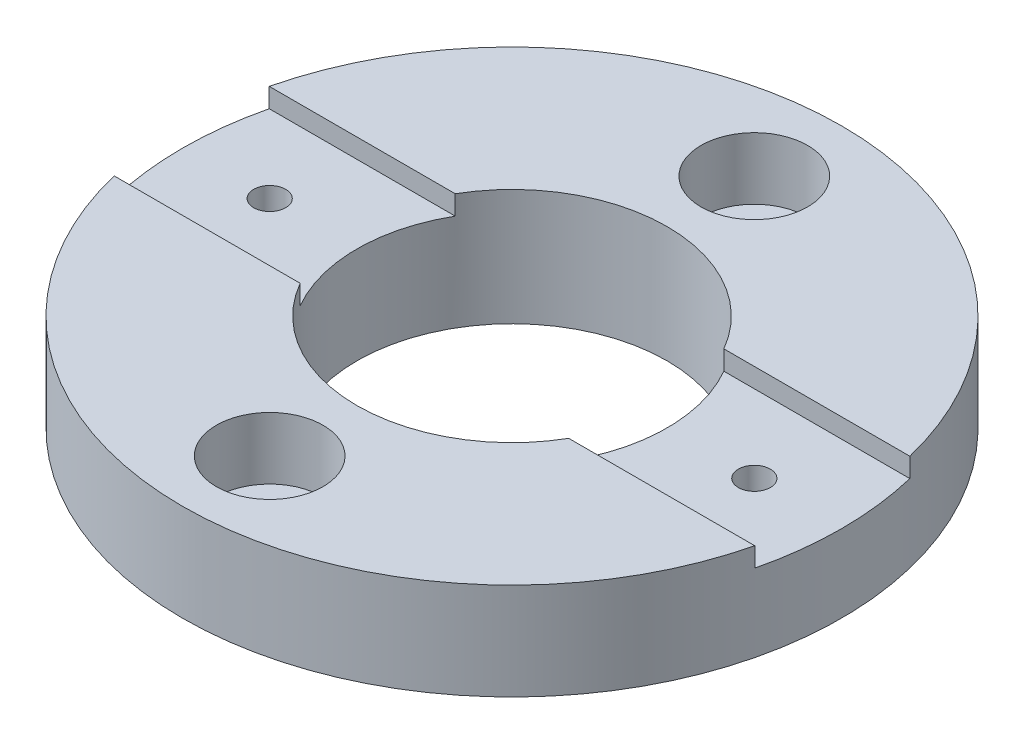
from build123d import *

# Parameters (mm, degrees)
HOLE_WIZARD_M6_1_D           = 6.6
HOLE_WIZARD_M6_1_CBORE_D     = 11
HOLE_WIZARD_M6_1_CBORE_DEPTH = 6.4
SKETCH_4_R                   = 16
CUT_EXTRUDE_1_DEPTH          = 67.543219038
EXTRUDE_1_DEPTH              = 10
SKETCH_6_W                   = 38
SKETCH_6_H                   = 16
CUT_EXTRUDE_2_DEPTH          = 10
CUT_EXTRUDE_3_DEPTH          = 74.810568349
CUT_EXTRUDE_3_DEPTH_BACK     = 74.810568349
SKETCH_7_R                   = 2
SKETCH_9_R                   = 20
CUT_EXTRUDE_5_DEPTH          = 34
SKETCH_10_W                  = 100
SKETCH_10_H                  = 16
CUT_EXTRUDE_6_DEPTH          = 12
HOLE_WIZARD_M4_1_D           = 3.3


with BuildPart() as part:
    # 草图1 → 旋转1 (revolve)
    with BuildSketch(Plane.XY, mode=Mode.PRIVATE) as revolve_1_sk:
        Polygon((0, 46), (34, 46), (34, 36), (18.4, 36), (18.4, 26), (17.492059993, 0), (0, 0), align=None)
    revolve(revolve_1_sk.sketch.rotate(Axis((0, 0, 0), (0, 1, 0)), 90), axis=Axis((0, 0, 0), (0, 1, 0)))

    # M6 六角凹头螺钉的柱形沉头孔1 (through all)
    with Locations(Plane(origin=(0, 46, 0), x_dir=(1, 0, 0), z_dir=(0, 1, 0))):
        with Locations((0, 25), (0, -25)):
            CounterBoreHole(HOLE_WIZARD_M6_1_D / 2, HOLE_WIZARD_M6_1_CBORE_D / 2, HOLE_WIZARD_M6_1_CBORE_DEPTH)

    # 草图4 → 切除-拉伸1 (cut, through all)
    with BuildSketch(Plane(origin=(0, 46, 0), x_dir=(1, 0, 0), z_dir=(0, 1, 0))):
        with Locations(Location((0, 0, 0), (0, 0, 270))):
            Circle(SKETCH_4_R)
    extrude(amount=-CUT_EXTRUDE_1_DEPTH, mode=Mode.SUBTRACT)

    # 草图5 → 凸台-拉伸1 (add)
    with BuildSketch(Plane(origin=(0, 46, 0), x_dir=(1, 0, 0), z_dir=(0, 1, 0))):
        with BuildLine():
            Line((33.045423284, -8), (13.856406461, -8))
            ThreePointArc((13.856406461, -8), (16, 0), (13.856406461, 8))
            Line((13.856406461, 8), (33.045423284, 8))
            ThreePointArc((33.045423284, 8), (34, 0), (33.045423284, -8))
        make_face()
        with BuildLine():
            Line((-33.045423284, 8), (-13.856406461, 8))
            ThreePointArc((-13.856406461, 8), (-16, 0), (-13.856406461, -8))
            Line((-13.856406461, -8), (-33.045423284, -8))
            ThreePointArc((-33.045423284, -8), (-34, 0), (-33.045423284, 8))
        make_face()
    extrude(amount=EXTRUDE_1_DEPTH)

    # 草图6 → 切除-拉伸2 (cut)
    with BuildSketch(Plane(origin=(0, 56, 0), x_dir=(1, 0, 0), z_dir=(0, 1, 0))):
        Rectangle(SKETCH_6_W, SKETCH_6_H)
    extrude(amount=-CUT_EXTRUDE_2_DEPTH, mode=Mode.SUBTRACT)

    # 草图7 → 切除-拉伸3 (cut, two sides: drawn at the far end of the back side and taken through both)
    with BuildSketch(Plane(origin=(0, 0, 0), x_dir=(0, 0, -1), z_dir=(1, 0, 0)).offset(-CUT_EXTRUDE_3_DEPTH_BACK)):
        with Locations((0, 50)):
            Circle(SKETCH_7_R)
    extrude(amount=CUT_EXTRUDE_3_DEPTH + CUT_EXTRUDE_3_DEPTH_BACK, mode=Mode.SUBTRACT)

    # 草图9 → 切除-拉伸5 (cut)
    with BuildSketch(Plane.XZ):
        Circle(SKETCH_9_R)
    extrude(amount=-CUT_EXTRUDE_5_DEPTH, mode=Mode.SUBTRACT)

    # 草图10 → 切除-拉伸6 (cut)
    with BuildSketch(Plane(origin=(0, 56, 0), x_dir=(1, 0, 0), z_dir=(0, 1, 0))):
        Rectangle(SKETCH_10_W, SKETCH_10_H)
    extrude(amount=-CUT_EXTRUDE_6_DEPTH, mode=Mode.SUBTRACT)

    # M4 螺纹孔1 (through all)
    with Locations(Plane(origin=(0, 46, 0), x_dir=(1, 0, 0), z_dir=(0, 1, 0))):
        with Locations((-25, 0), (25, 0)):
            Hole(HOLE_WIZARD_M4_1_D / 2)


solid = part.part
